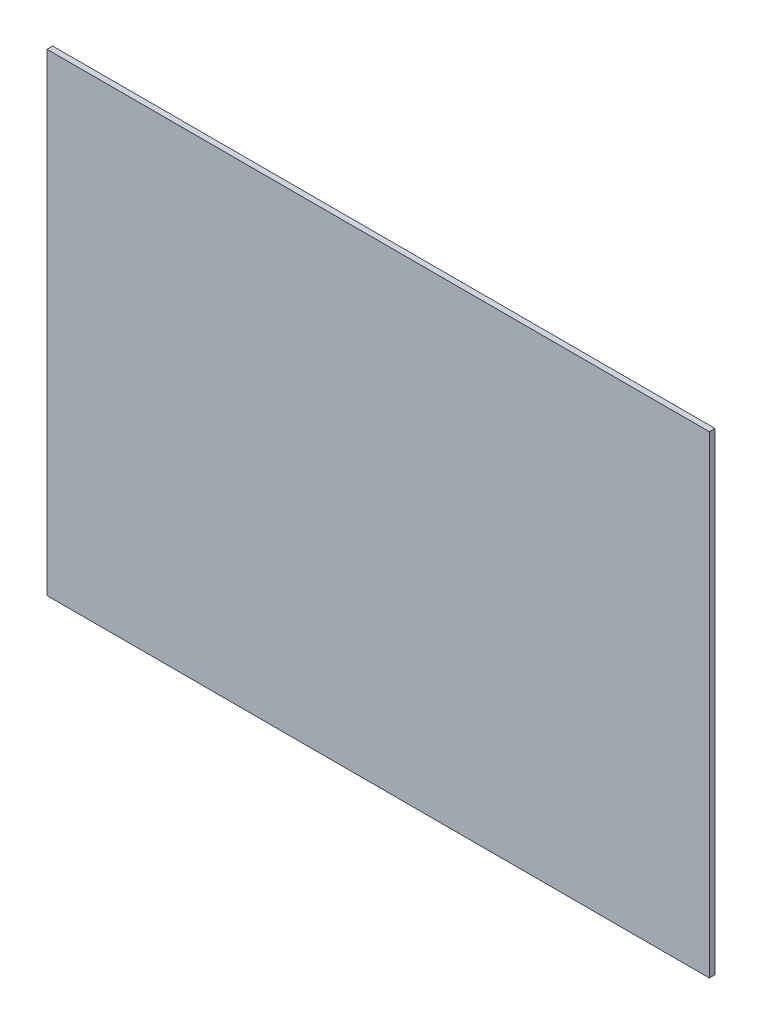
from build123d import *

# Parameters (mm, degrees)
SKETCH1_W           = 700
SKETCH1_H           = 500
BOSS_EXTRUDE1_DEPTH = 3


with BuildPart() as part:
    # Sketch1 → Boss-Extrude1 (new, symmetric)
    with BuildSketch(Plane.XY):
        Rectangle(SKETCH1_W, SKETCH1_H)
    extrude(amount=BOSS_EXTRUDE1_DEPTH, both=True)


solid = part.part
